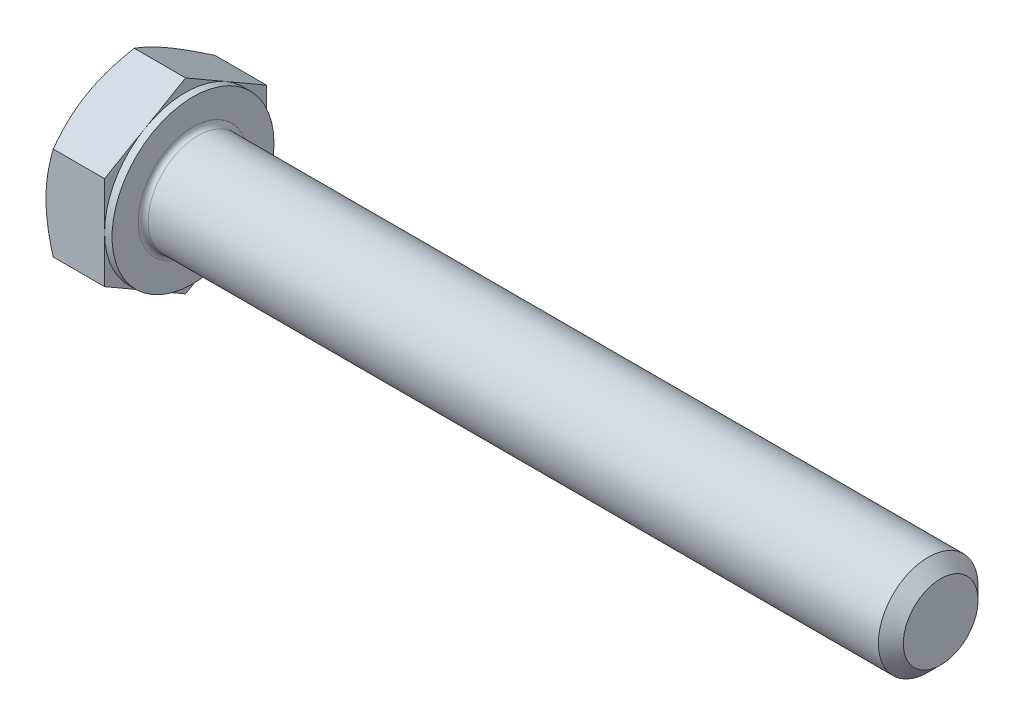
from build123d import *

# Parameters (mm, degrees)
BASE_EXTRUDE_DEPTH = 5.3
SKETCH4_W          = 0.6
SKETCH4_H          = 11.005553499
CHAMFER_2_SIZE     = 1
FILLET_2_R         = 0.4


with BuildPart() as part:
    # Sketch1 → Base-Extrude (new body)
    with BuildSketch(Plane(origin=(0, 0, 0), x_dir=(0, 0, -1), z_dir=(1, 0, 0))):
        Polygon((6.5, 3.75277675), (6.5, -3.75277675), (0, -7.505553499), (-6.5, -3.75277675), (-6.5, 3.75277675), (0, 7.505553499), align=None)
    extrude(amount=BASE_EXTRUDE_DEPTH)

    # Sketch2 → Boss-Revolve1 (revolve)
    with BuildSketch(Plane.XY, mode=Mode.PRIVATE) as boss_revolve1_sk:
        Polygon((0, 0), (65.3, 0), (65.3, 2.9175), (65.3, 4), (7.791693541, 4), (0, 4), align=None)
    revolve(boss_revolve1_sk.sketch.rotate(Axis((0, 0, 0), (1, 0, 0)), 90), axis=Axis((0, 0, 0), (1, 0, 0)))

    # Sketch3 → Cut-Revolve1 (revolve, cut)
    with BuildSketch(Plane.XY):
        Polygon((0, 6.5), (3.46730793, 12.505553499), (3.46730793, 17.505553499), (-10, 17.505553499), (-10, 6.5), align=None)
    revolve(axis=Axis((0, 0, 0), (1, 0, 0)), mode=Mode.SUBTRACT)

    # Sketch5 → Cut-Revolve2 (revolve, cut)
    with BuildSketch(Plane.XY):
        Polygon((5.3, 6.5), (1.83269207, 12.505553499), (1.83269207, 17.505553499), (11.83269207, 17.505553499), (11.83269207, 6.5), align=None)
    revolve(axis=Axis((0, 0, 0), (1, 0, 0)), mode=Mode.SUBTRACT)

    # Sketch4 → Cut-Revolve3 (revolve, cut)
    with BuildSketch(Plane.XY, mode=Mode.PRIVATE) as cut_revolve3_sk:
        with Locations((5, 12.00277675)):
            Rectangle(SKETCH4_W, SKETCH4_H)
    revolve(cut_revolve3_sk.sketch.rotate(Axis((0, 0, 0), (1, 0, 0)), 270), axis=Axis((0, 0, 0), (1, 0, 0)), mode=Mode.SUBTRACT)

    # Chamfer 2
    chamfer_2_edges = [part.edges().sort_by_distance(p)[0] for p in [
        (65.3, 0, -4),
    ]]
    chamfer(chamfer_2_edges, length=CHAMFER_2_SIZE)

    # Fillet 2
    fillet_2_edges = [part.edges().sort_by_distance(p)[0] for p in [
        (5.3, 0, -4),
    ]]
    fillet(fillet_2_edges, radius=FILLET_2_R)


solid = part.part
